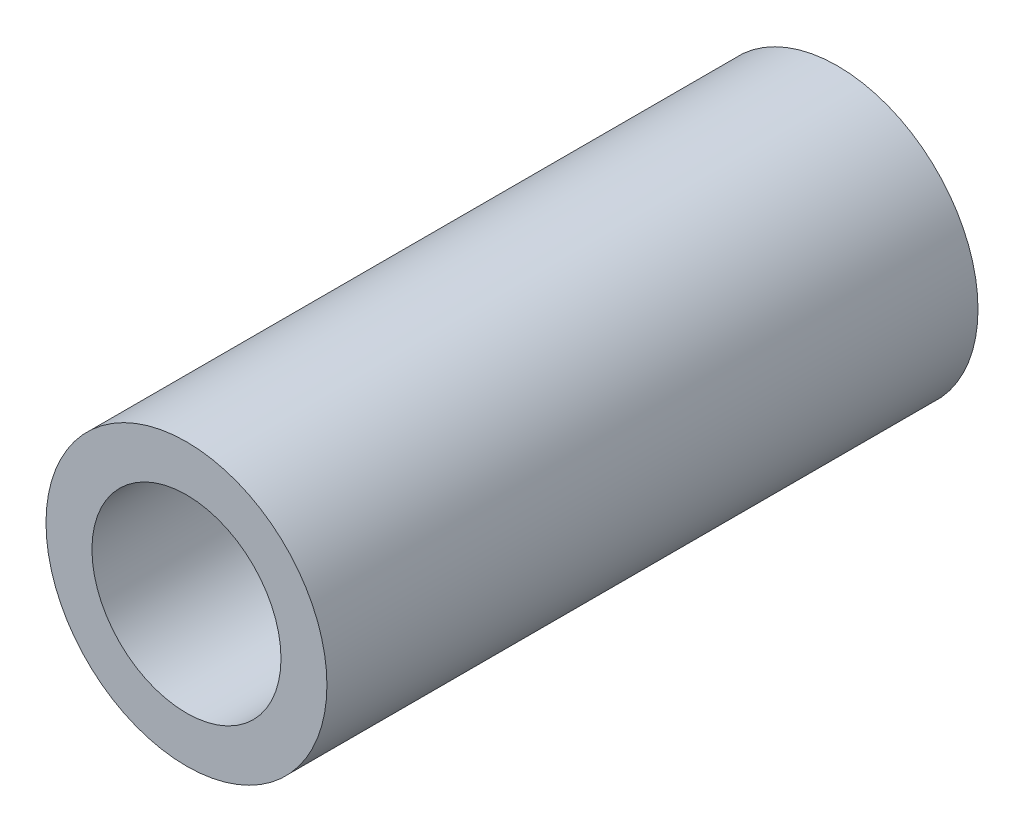
from build123d import *

# Parameters (mm, degrees)
SKETCH1_R           = 6.85
SKETCH1_R_2         = 4.61
BOSS_EXTRUDE1_DEPTH = 15.875


with BuildPart() as part:
    # Sketch1 → Boss-Extrude1 (new, symmetric)
    with BuildSketch(Plane.XY):
        Circle(SKETCH1_R)
        Circle(SKETCH1_R_2, mode=Mode.SUBTRACT)
    extrude(amount=BOSS_EXTRUDE1_DEPTH, both=True)


solid = part.part
